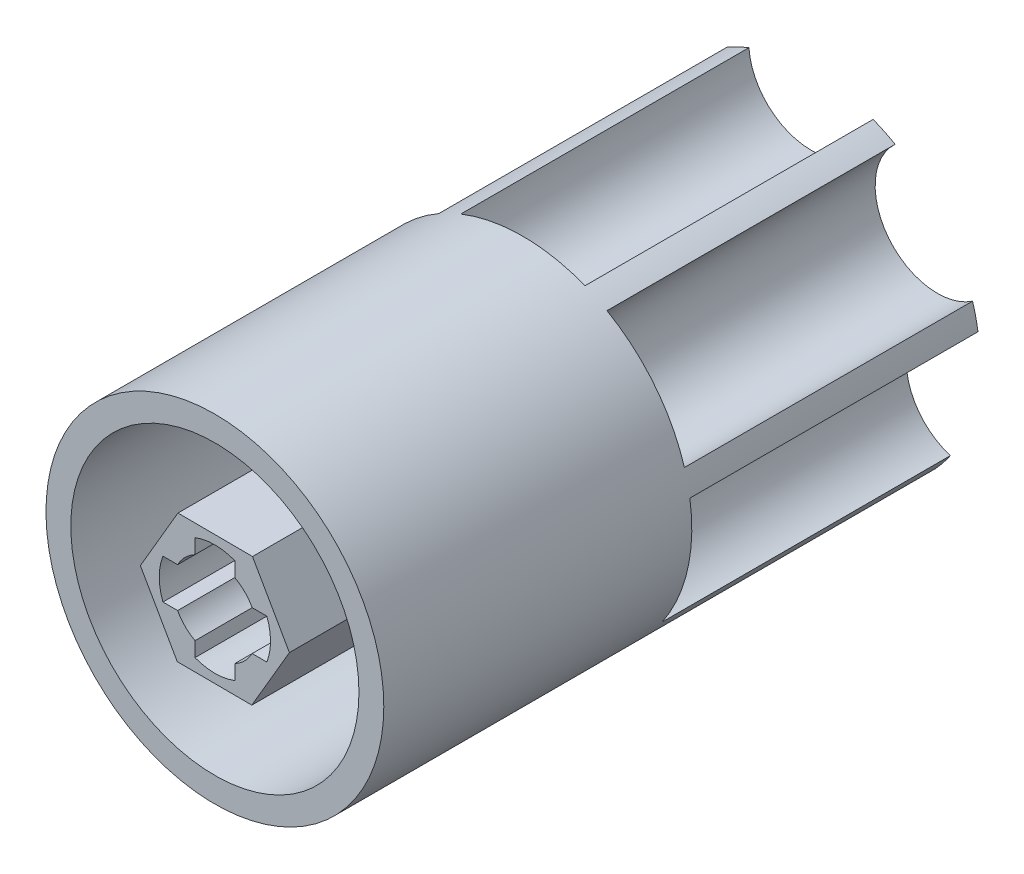
from build123d import *
from build123d.topology import SkipClean

# Parameters (mm, degrees)
SKETCH_1_R        = 34
SKETCH_1_R_2      = 29
EXTRUDE_1_DEPTH   = 60
EXTRUDE_1_2_DEPTH = 60
EXTRUDE_START     = -60
EXTRUDE_2_DEPTH   = 60
EXTRUDE_START_2   = -2
SKETCH_4_R        = 34
EXTRUDE_3_DEPTH   = 2


with BuildPart() as part:
    # 草图1 → 凸台-拉伸1 (new body)
    with BuildSketch(Plane.XY):
        Circle(SKETCH_1_R)
        Circle(SKETCH_1_R_2, mode=Mode.SUBTRACT)
    extrude(amount=EXTRUDE_1_DEPTH)



with BuildPart() as body_2:
    # 草图1 → Extrude 1 2 (new body)
    with BuildSketch(Plane.XY):
        Polygon((-15, 0.078188502), (-7.567713229, -12.951286806), (7.432286771, -13.029475308), (15, -0.078188502), (7.567713229, 12.951286806), (-7.432286771, 13.029475308), align=None)
        with BuildLine():
            ThreePointArc((-10.461357464, 4), (-11.2, 0), (-10.461357464, -4))
            Line((-10.461357464, -4), (-7.5, -4))
            ThreePointArc((-7.5, -4), (-6.01040764, -6.01040764), (-4, -7.5))
            Line((-4, -7.5), (-4, -10.461357464))
            ThreePointArc((-4, -10.461357464), (0, -11.2), (4, -10.461357464))
            Line((4, -10.461357464), (4, -7.5))
            ThreePointArc((4, -7.5), (6.01040764, -6.01040764), (7.5, -4))
            Line((7.5, -4), (10.461357464, -4))
            ThreePointArc((10.461357464, -4), (11.2, 0), (10.461357464, 4))
            Line((10.461357464, 4), (7.5, 4))
            ThreePointArc((7.5, 4), (6.01040764, 6.01040764), (4, 7.5))
            Line((4, 7.5), (4, 10.461357464))
            ThreePointArc((4, 10.461357464), (0, 11.2), (-4, 10.461357464))
            Line((-4, 10.461357464), (-4, 7.5))
            ThreePointArc((-4, 7.5), (-6.01040764, 6.01040764), (-7.5, 4))
            Line((-7.5, 4), (-10.461357464, 4))
        make_face(mode=Mode.SUBTRACT)
    extrude(amount=EXTRUDE_1_2_DEPTH)


with BuildPart() as part_1:
    add(part.part)

    add(body_2.part)  # 凸台-拉伸2 merges body 2
    # 草图2 → 凸台-拉伸2 (add)
    with BuildSketch(Plane.XY.offset(EXTRUDE_START)):
        with BuildLine():
            ThreePointArc((16.926969134, 29.486907535), (14.75204713, 30.632941509), (12.5, 31.618823508))
            ThreePointArc((12.5, 31.618823508), (0, 20), (-12.5, 31.618823508))
            ThreePointArc((-12.5, 31.618823508), (-14.75204713, 30.632941509), (-16.926969134, 29.486907535))
            ThreePointArc((-16.926969134, 29.486907535), (-15.636629649, 12.469796037), (-32.51421418, 9.941120473))
            ThreePointArc((-32.51421418, 9.941120473), (-33.147549014, 7.565711755), (-33.607585262, 5.150748765))
            ThreePointArc((-33.607585262, 5.150748765), (-19.498558244, -4.450418679), (-28.044561913, -19.22244904))
            ThreePointArc((-28.044561913, -19.22244904), (-26.582270404, -21.198653263), (-24.981004219, -23.064028881))
            ThreePointArc((-24.981004219, -23.064028881), (-8.677674782, -18.019377358), (-2.456782521, -33.911122359))
            ThreePointArc((-2.456782521, -33.911122359), (0, -34), (2.456782521, -33.911122359))
            ThreePointArc((2.456782521, -33.911122359), (8.677674782, -18.019377358), (24.981004219, -23.064028881))
            ThreePointArc((24.981004219, -23.064028881), (26.582270404, -21.198653263), (28.044561913, -19.22244904))
            ThreePointArc((28.044561913, -19.22244904), (19.498558244, -4.450418679), (33.607585262, 5.150748765))
            ThreePointArc((33.607585262, 5.150748765), (33.147549014, 7.565711755), (32.51421418, 9.941120473))
            ThreePointArc((32.51421418, 9.941120473), (15.636629649, 12.469796037), (16.926969134, 29.486907535))
        make_face()
        with BuildLine():
            Line((-10.461357464, -4), (-7.5, -4))
            ThreePointArc((-7.5, -4), (-6.01040764, -6.01040764), (-4, -7.5))
            Line((-4, -7.5), (-4, -10.461357464))
            ThreePointArc((-4, -10.461357464), (0, -11.2), (4, -10.461357464))
            Line((4, -10.461357464), (4, -7.5))
            ThreePointArc((4, -7.5), (6.01040764, -6.01040764), (7.5, -4))
            Line((7.5, -4), (10.461357464, -4))
            ThreePointArc((10.461357464, -4), (11.2, 0), (10.461357464, 4))
            Line((10.461357464, 4), (7.5, 4))
            ThreePointArc((7.5, 4), (6.01040764, 6.01040764), (4, 7.5))
            Line((4, 7.5), (4, 10.461357464))
            ThreePointArc((4, 10.461357464), (0, 11.2), (-4, 10.461357464))
            Line((-4, 10.461357464), (-4, 7.5))
            ThreePointArc((-4, 7.5), (-6.01040764, 6.01040764), (-7.5, 4))
            Line((-7.5, 4), (-10.461357464, 4))
            ThreePointArc((-10.461357464, 4), (-11.2, 0), (-10.461357464, -4))
        make_face(mode=Mode.SUBTRACT)
    extrude(amount=EXTRUDE_2_DEPTH)

    # 草图4 → 凸台-拉伸3 (add)
    with SkipClean():  # the faces are left unmerged after this step: merging them gives an invalid solid
        with BuildSketch(Plane.XY.offset(EXTRUDE_START_2)):
            with Locations(Location((0, 0, 0), (0, 0, 171.286564556))):
                Circle(SKETCH_4_R)
            with BuildLine():
                ThreePointArc((21.649435664, -19.295127245), (22.673112992, -18.081204254), (23.628810764, -16.813069377))
                ThreePointArc((23.628810764, -16.813069377), (19.498558244, -4.450418679), (28.583740291, 4.895895317))
                ThreePointArc((28.583740291, 4.895895317), (28.272909453, 6.453107085), (27.877309497, 7.990970854))
                ThreePointArc((27.877309497, 7.990970854), (15.636629649, 12.469796037), (13.993905477, 25.400208848))
                ThreePointArc((13.993905477, 25.400208848), (12.582628434, 26.128097169), (11.133625585, 26.777647046))
                ThreePointArc((11.133625585, 26.777647046), (0, 20), (-11.133625585, 26.777647046))
                ThreePointArc((-11.133625585, 26.777647046), (-12.582628434, 26.128097169), (-13.993905477, 25.400208848))
                ThreePointArc((-13.993905477, 25.400208848), (-15.636629649, 12.469796037), (-27.877309497, 7.990970854))
                ThreePointArc((-27.877309497, 7.990970854), (-28.272909453, 6.453107085), (-28.583740291, 4.895895317))
                ThreePointArc((-28.583740291, 4.895895317), (-19.498558244, -4.450418679), (-23.628810764, -16.813069377))
                ThreePointArc((-23.628810764, -16.813069377), (-22.673112992, -18.081204254), (-21.649435664, -19.295127245))
                ThreePointArc((-21.649435664, -19.295127245), (-8.677674782, -18.019377358), (-1.587335586, -28.956525443))
                ThreePointArc((-1.587335586, -28.956525443), (0, -29), (1.587335586, -28.956525443))
                ThreePointArc((1.587335586, -28.956525443), (8.677674782, -18.019377358), (21.649435664, -19.295127245))
            make_face(mode=Mode.SUBTRACT)
        extrude(amount=EXTRUDE_3_DEPTH)


solid = part_1.part
